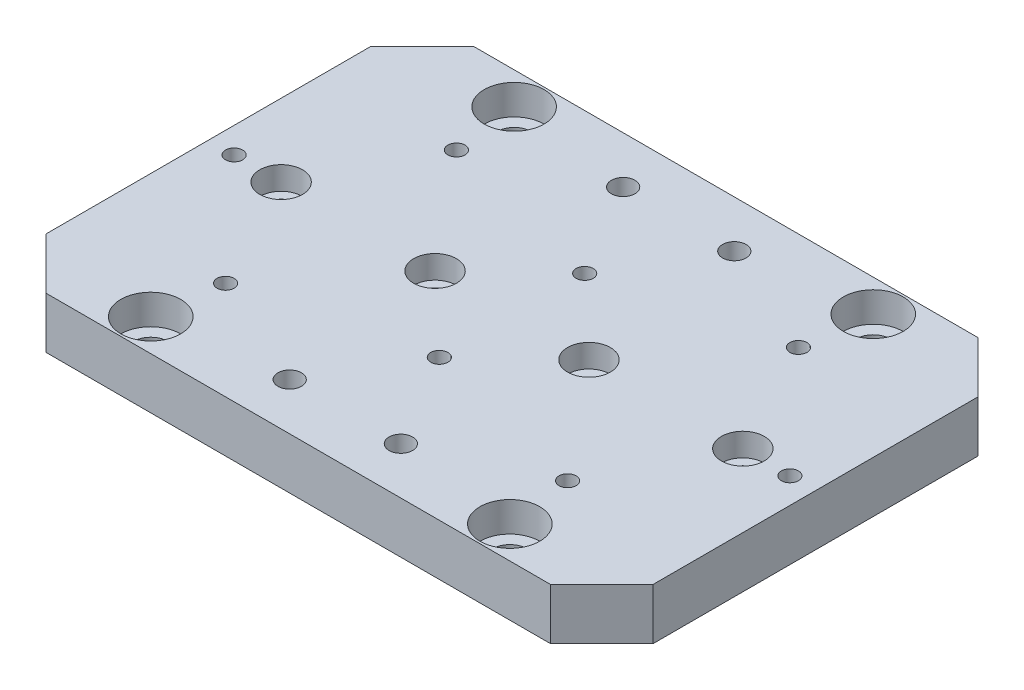
SolidWorks part; units mm, degrees
material "A6061"
ref_plane "前视基准面" through (0, 0, 0) normal (0, 0, 1) x (1, 0, 0)
ref_plane "上视基准面" through (0, 0, 0) normal (0, 1, 0) x (1, 0, 0)
ref_plane "右视基准面" through (0, 0, 0) normal (1, 0, 0) x (0, 0, -1)
sketch "Sketch1" plane through (0, 0, 0) normal (0, 1, 0) x (1, 0, 0)
  line L1 (71, -50) -> (-71, -50)
  line L2 (71, -50) -> (71, 50)
  line L3 (71, 50) -> (-71, 50)
  line L4 (-71, -50) -> (-71, 50)
  line L5 (71, -50) -> (-71, 50) construction
  line L6 (71, 50) -> (-71, -50) construction
  point P0 (0, 0)
  dimension "D1" = 142
  dimension "D2" = 100
extrude "Extrude1" add sketch "Sketch1" along normal blind 12
hole_wizard "CBORE for M5 Hex Socket Head Cap Screw1" positions "Sketch3" profile "Sketch2" counterbore size "M5" standard "ISO" end condition through all
sketch "Sketch3" plane through (0, 0, 0) normal (0, -1, 0) x (-1, 0, 0)
  line L0 (-13, 39) -> (13, 39) construction
  line L1 (13, 39) -> (13, -39) construction
  line L2 (13, -39) -> (-13, -39) construction
  line L3 (-13, -39) -> (-13, 39) construction
  line L5 (0, 0) -> (0, 39) construction
  line L7 (0, 0) -> (13, 0) construction
  point P0 (-13, -39)
  point P2 (13, 39)
  point P4 (-13, 39)
  point P6 (13, -39)
  dimension "D1" = 78
  dimension "D2" = 26
sketch "Sketch2" plane through (13, 0, 39) normal (1, 0, 0) x (0, 0, -1)
  line L0 (0, 0) -> (0, 12)
  line L1 (0, 12) -> (2.75, 12)
  line L3 (2.75, 12) -> (2.75, 5.4)
  line L4 (2.75, 5.4) -> (5, 5.4)
  line L5 (5, 5.4) -> (5, 0)
  line L7 (5, 0) -> (0, 0)
  line L11 (0, -6.35) -> (0, 107.95) construction
  dimension "通孔孔直径" = 5.5
  dimension "通孔孔深度" = 12
  dimension "柱形沉头孔直径" = 10
  dimension "柱形沉头孔深度" = 5.4
hole_wizard "CBORE for M5 Hex Socket Head Cap Screw2" positions "Sketch5" profile "Sketch4" counterbore size "M5" standard "ISO" end condition through all
sketch "Sketch5" plane through (0, 12, 0) normal (0, 1, 0) x (1, 0, 0)
  point P0 (-54, 0)
  point P9 (54, 0)
  point P33 (-18, 0)
  point P36 (18, 0)
sketch "Sketch4" plane through (-54, 12, 0) normal (1, 0, 0) x (0, 0, 1)
  line L0 (0, 0) -> (0, 12)
  line L1 (0, 12) -> (2.75, 12)
  line L3 (2.75, 12) -> (2.75, 5.4)
  line L4 (2.75, 5.4) -> (5, 5.4)
  line L5 (5, 5.4) -> (5, 0)
  line L7 (5, 0) -> (0, 0)
  line L11 (0, -6.35) -> (0, 107.95) construction
  dimension "通孔孔直径" = 5.5
  dimension "通孔孔深度" = 12
  dimension "柱形沉头孔直径" = 10
  dimension "柱形沉头孔深度" = 5.4
hole_wizard "大小mm 暗销孔0" positions "Sketch7" profile "Sketch6" hole size "Ø4.0" standard "GB" end condition through all
sketch "Sketch7" plane through (0, 12, 0) normal (0, 1, 0) x (1, 0, 0)
  line L3 (-40, 27) -> (40, 27) construction
  line L4 (40, 27) -> (40, -27) construction
  line L7 (0, 0) -> (40, 0) construction
  line L8 (0, 0) -> (0, 27) construction
  line L9 (71, -25) -> (-71, -25) construction
  point P16 (-40, 27)
  point P18 (40, 27)
  point P20 (40, -27)
  point P22 (-40, -27)
  dimension "D1" = 2
  dimension "D2" = 80
sketch "Sketch6" plane through (-40, 12, -27) normal (1, 0, 0) x (0, 0, 1)
  line L0 (0, 0) -> (0, 12)
  line L1 (0, 12) -> (2, 12)
  line L2 (2, 12) -> (2, 0)
  line L5 (2, 0) -> (0, 0)
  line L11 (0, -6.35) -> (0, 107.95) construction
  dimension "通孔孔直径" = 4
  dimension "通孔孔深度" = 12
chamfer "Chamfer1" distance 12 angle 45 4 edges at (-71, 6, -50) (-71, 6, 50) (71, 6, -50) (71, 6, 50)
hole_wizard "Ø4.0 mm Dowel Holes1" positions "Sketch9" profile "Sketch8" hole size "Ø4.0" standard "GB" end condition through all
sketch "Sketch9" plane through (0, 12, 0) normal (0, 1, 0) x (1, 0, 0)
  line L0 (-67.5, 0) -> (-62.5, 0) construction
  arc A0 (-65.5, 2) -> (-65.5, -2) centre (-65.5, 0) ccw construction
  arc A1 (-64.5, -2) -> (-64.5, 2) centre (-64.5, 0) ccw construction
  point P10 (-65, 0)
  point P12 (65, 0)
sketch "Sketch8" plane through (-65, 12, 0) normal (1, 0, 0) x (0, 0, 1)
  line L0 (0, 0) -> (0, 12)
  line L1 (0, 12) -> (2, 12)
  line L2 (2, 12) -> (2, 0)
  line L5 (2, 0) -> (0, 0)
  line L11 (0, -6.35) -> (0, 107.95) construction
  dimension "通孔孔直径" = 4
  dimension "通孔孔深度" = 12
hole_wizard "Ø8.0 mm Dowel Holes1" positions "Sketch11" profile "Sketch12" hole size "Ø8.0" standard "GB" end condition through all
sketch "Sketch11" plane through (0, 12, 0) normal (0, 1, 0) x (1, 0, 0)
  point P0 (-42, 42.5)
  point P3 (42, 42.5)
  point P6 (42, -42.5)
  point P9 (-42, -42.5)
sketch "Sketch12" plane through (-42, 12, -42.5) normal (1, 0, 0) x (0, 0, 1)
  line L0 (0, 0) -> (0, 12)
  line L1 (0, 12) -> (4, 12)
  line L2 (4, 12) -> (4, 0)
  line L5 (4, 0) -> (0, 0)
  line L11 (0, -6.35) -> (0, 107.95) construction
  dimension "通孔孔直径" = 8
  dimension "通孔孔深度" = 12
sketch "Sketch13" plane through (0, 12, 0) normal (0, 1, 0) x (1, 0, 0)
  circle A0 centre (-42, -42.5) radius 7
  circle A1 centre (42, -42.5) radius 7
  circle A2 centre (-42, 42.5) radius 7
  circle A3 centre (42, 42.5) radius 7
  dimension "D1" = 14
extrude "Extrude2" cut sketch "Sketch13" against normal blind 7
hole_wizard "Ø4.0 mm Dowel Holes2" positions "Sketch15" profile "Sketch14" hole size "Ø4.0" standard "GB" end condition through all
sketch "Sketch15" plane through (0, 0, 0) normal (0, -1, 0) x (-1, 0, 0)
  point P0 (0, 17)
  point P3 (0, -17)
sketch "Sketch14" plane through (0, 0, -17) normal (1, 0, 0) x (0, 0, -1)
  line L0 (0, 0) -> (0, 12)
  line L1 (0, 12) -> (2, 12)
  line L2 (2, 12) -> (2, 0)
  line L5 (2, 0) -> (0, 0)
  line L11 (0, -6.35) -> (0, 107.95) construction
  dimension "通孔孔直径" = 4
  dimension "通孔孔深度" = 12
